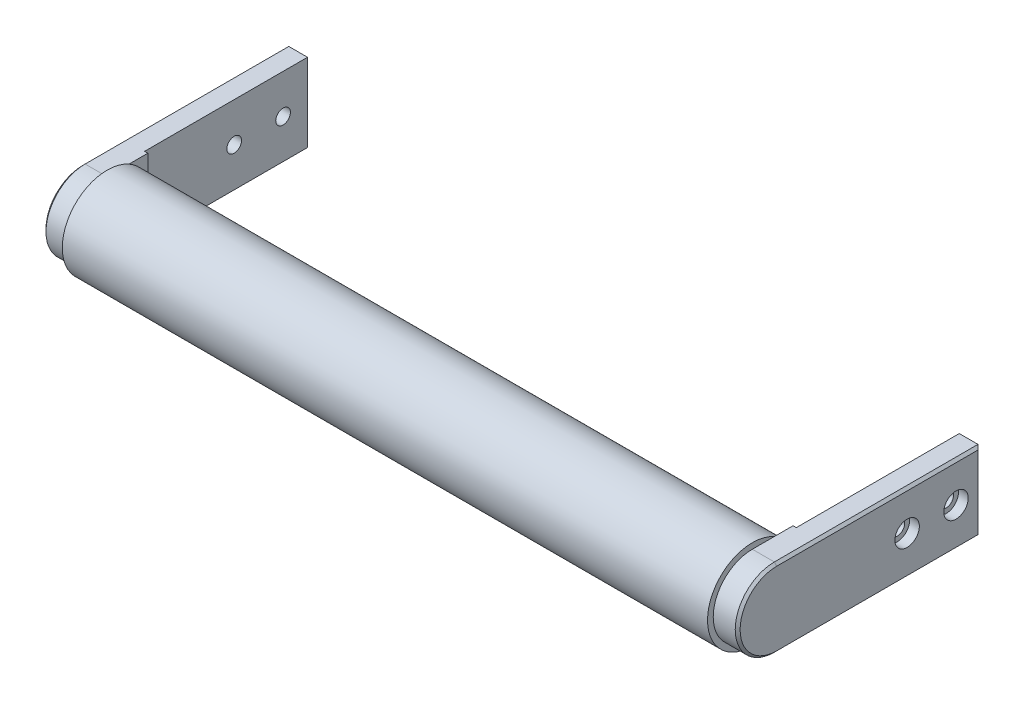
SolidWorks part; units mm, degrees
material "延性铁"
ref_plane "前视基准面" through (0, 0, 0) normal (0, 0, 1) x (1, 0, 0)
ref_plane "上视基准面" through (0, 0, 0) normal (0, 1, 0) x (1, 0, 0)
ref_plane "右视基准面" through (0, 0, 0) normal (1, 0, 0) x (0, 0, -1)
sketch "草图1" plane through (0, 0, 0) normal (1, 0, 0) x (0, 0, -1)
  line L1 (-62.5, 24) -> (62.5, 24)
  line L2 (-62.5, 24) -> (-62.5, -24) construction
  line L3 (-62.5, -24) -> (62.5, -24)
  line L4 (62.5, 24) -> (62.5, -24)
  line L5 (-62.5, 24) -> (62.5, -24) construction
  line L6 (-62.5, -24) -> (62.5, 24) construction
  arc A0 (-62.5, 24) -> (-62.5, -24) centre (-62.5, 0) ccw
  point P0 (0, 0)
  dimension "D1" = 48
  dimension "D2" = 125
extrude "凸台-拉伸1" add sketch "草图1" along normal blind 15
sketch "草图2" plane through (0, 0, 0) normal (-1, 0, 0) x (0, 0, 1)
  circle A0 centre (62.5, 0) radius 27.5
  dimension "D1" = 55
extrude "凸台-拉伸2" add sketch "草图2" along normal blind 396
hole_wizard "打孔尺寸(%根据)内六角花形圆柱头螺钉1" positions "草图3" profile "草图4" counterbore size "M8" standard "GB" end condition through all
sketch "草图3" plane through (15, 0, 0) normal (1, 0, 0) x (0, 0, -1)
  line L0 (62.5, 0) -> (-4.2393, 0) construction
  line L1 (62.5, -24) -> (62.5, 24) construction
  point P0 (17.5, 0)
  point P2 (47.5, 0)
  dimension "D1" = 15
  dimension "D2" = 30
sketch "草图4" plane through (15, 0, -17.5) normal (0, 1, 0) x (0, 0, -1)
  line L0 (0, 0) -> (0, 426)
  line L1 (0, 426) -> (4.5, 426)
  line L3 (4.5, 426) -> (4.5, 6)
  line L4 (4.5, 6) -> (7.5, 6)
  line L5 (7.5, 6) -> (7.5, 0)
  line L7 (7.5, 0) -> (0, 0)
  line L11 (0, -6.35) -> (0, 107.95) construction
  dimension "通孔孔直径" = 9
  dimension "通孔孔深度" = 426
  dimension "柱形沉头孔直径" = 15
  dimension "柱形沉头孔深度" = 6
chamfer "倒角1" distance 1.5 angle 45 4 edges at (15, 0, -62.5) (15, -24, 0) (15, 0, 86.5) (15, 24, 0)
ref_plane "基准面1" through (-198, 0, 0) normal (-1, 0, 0) x (0, 0, 1)
mirror "镜向1" about plane through (-198, 0, 0) normal (-1, 0, 0) of "倒角1", "凸台-拉伸1", "打孔尺寸(%根据)内六角花形圆柱头螺钉1"
sketch "草图5" plane through (0, 24, 0) normal (0, 1, 0) x (1, 0, 0)
  line L1 (-396, 62.5) -> (-398, 62.5)
  line L2 (-396, 62.5) -> (-396, -37.5)
  line L3 (-396, -37.5) -> (-398, -37.5)
  line L4 (-398, 62.5) -> (-398, -37.5)
  line L5 (0, 62.5) -> (2, 62.5)
  line L6 (0, 62.5) -> (0, -37.5)
  line L7 (0, -37.5) -> (2, -37.5)
  line L8 (2, 62.5) -> (2, -37.5)
  dimension "D1" = 100
  dimension "D2" = 2
  dimension "D3" = 2
extrude "切除-拉伸1" cut sketch "草图5" against normal through all
